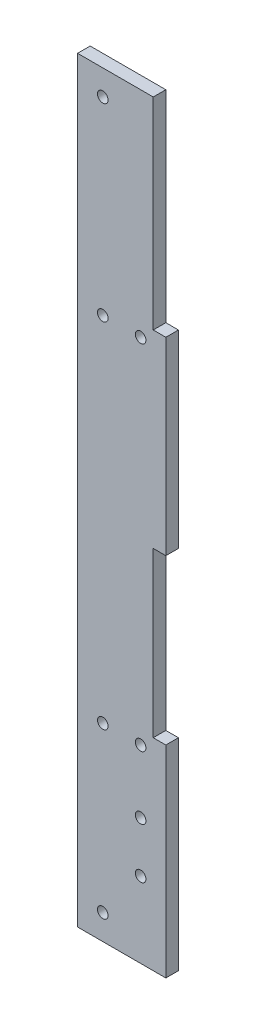
from build123d import *

# Parameters (mm, degrees)
SKETCH1_R           = 2.1
BOSS_EXTRUDE1_DEPTH = 5


with BuildPart() as part:
    # Sketch1 → Boss-Extrude1 (new body)
    with BuildSketch(Plane.XY):
        Polygon((30, 300), (30, 220), (35, 220), (35, 145), (30, 145), (30, 80), (35, 80), (35, 0), (0, 0), (0, 300), align=None)
        with Locations((25, 215)):
            Circle(SKETCH1_R, mode=Mode.SUBTRACT)
        with Locations((10, 215)):
            Circle(SKETCH1_R, mode=Mode.SUBTRACT)
        with Locations((25, 75)):
            Circle(SKETCH1_R, mode=Mode.SUBTRACT)
        with Locations((10, 75)):
            Circle(SKETCH1_R, mode=Mode.SUBTRACT)
        with Locations((10, 290)):
            Circle(SKETCH1_R, mode=Mode.SUBTRACT)
        with Locations((10, 10)):
            Circle(SKETCH1_R, mode=Mode.SUBTRACT)
        with Locations((25, 30)):
            Circle(SKETCH1_R, mode=Mode.SUBTRACT)
        with Locations((25, 50)):
            Circle(SKETCH1_R, mode=Mode.SUBTRACT)
    extrude(amount=BOSS_EXTRUDE1_DEPTH)


solid = part.part
